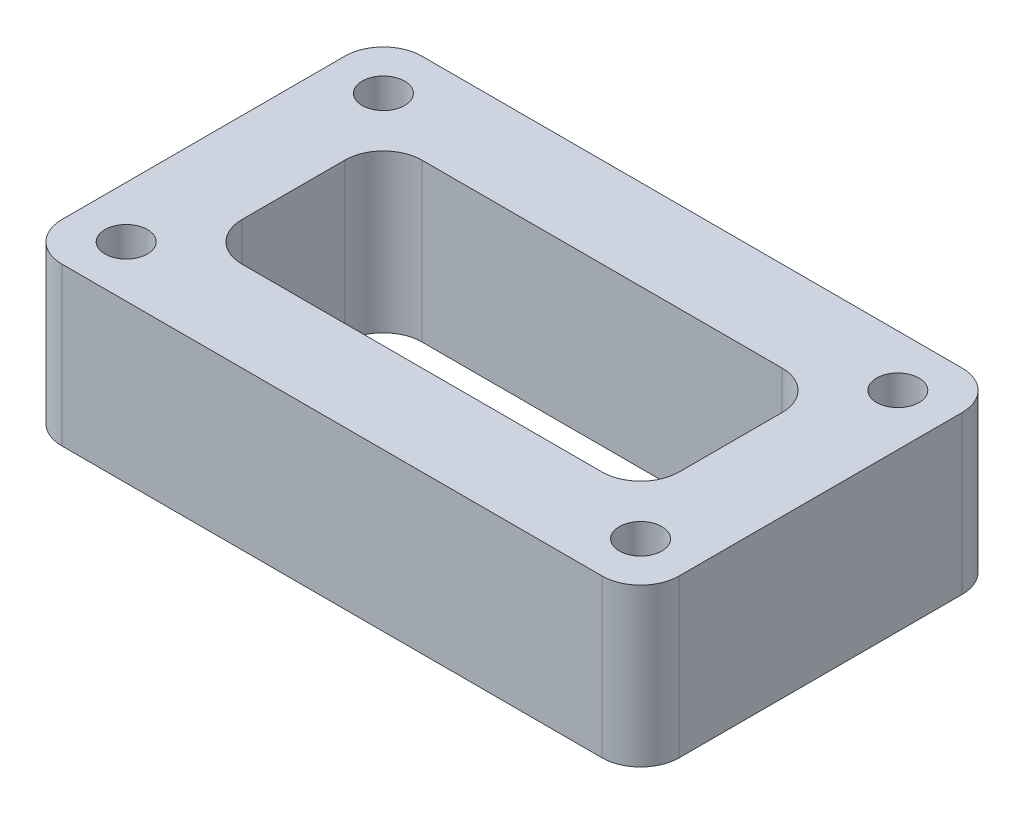
from build123d import *

# Parameters (mm, degrees)
SKETCH_1_R      = 1.65
EXTRUDE_1_DEPTH = 12.25


with BuildPart() as part:
    # 草图1 → 凸台-拉伸1 (new body)
    with BuildSketch(Plane(origin=(0, 0, 0), x_dir=(1, 0, 0), z_dir=(0, 1, 0))):
        with BuildLine():
            Line((-24, -11), (-24, 11))
            ThreePointArc((-24, 11), (-23.121320344, 13.121320344), (-21, 14))
            Line((-21, 14), (21, 14))
            ThreePointArc((21, 14), (23.121320344, 13.121320344), (24, 11))
            Line((24, 11), (24, -11))
            ThreePointArc((24, -11), (23.121320344, -13.121320344), (21, -14))
            Line((21, -14), (-21, -14))
            ThreePointArc((-21, -14), (-23.121320344, -13.121320344), (-24, -11))
        make_face()
        with Locations(Location((-20, 10, 0), (0, 0, 270))):
            Circle(SKETCH_1_R, mode=Mode.SUBTRACT)
        with Locations(Location((-20, -10, 0), (0, 0, 270))):
            Circle(SKETCH_1_R, mode=Mode.SUBTRACT)
        with Locations(Location((20, -10, 0), (0, 0, 270))):
            Circle(SKETCH_1_R, mode=Mode.SUBTRACT)
        with Locations(Location((20, 10, 0), (0, 0, 270))):
            Circle(SKETCH_1_R, mode=Mode.SUBTRACT)
        with BuildLine():
            Line((-17, -4), (-17, 4))
            ThreePointArc((-17, 4), (-16.121320344, 6.121320344), (-14, 7))
            Line((-14, 7), (14, 7))
            ThreePointArc((14, 7), (16.121320344, 6.121320344), (17, 4))
            Line((17, 4), (17, -4))
            ThreePointArc((17, -4), (16.121320344, -6.121320344), (14, -7))
            Line((14, -7), (-14, -7))
            ThreePointArc((-14, -7), (-16.121320344, -6.121320344), (-17, -4))
        make_face(mode=Mode.SUBTRACT)
    extrude(amount=EXTRUDE_1_DEPTH)


solid = part.part
